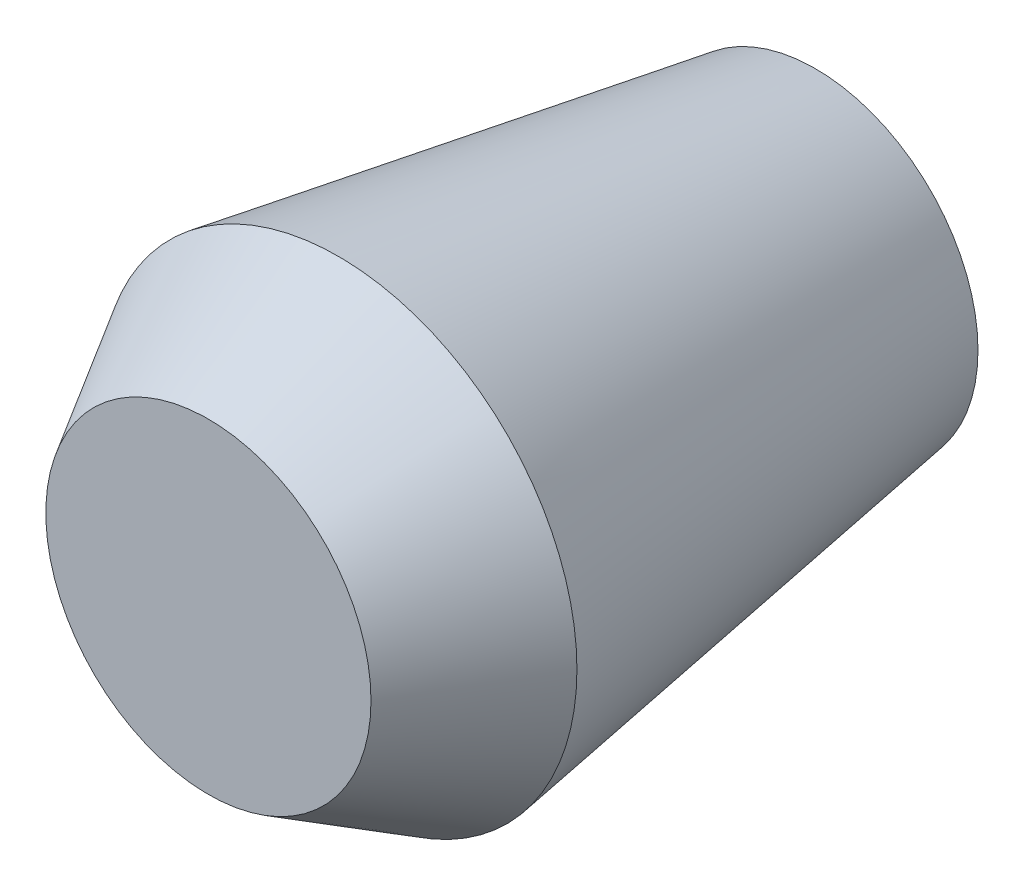
SolidWorks part; units mm, degrees
ref_plane "Front Plane" through (0, 0, 0) normal (0, 0, 1) x (1, 0, 0)
ref_plane "Top Plane" through (0, 0, 0) normal (0, 1, 0) x (1, 0, 0)
ref_plane "Right Plane" through (0, 0, 0) normal (1, 0, 0) x (0, 0, -1)
other "Configuration Table"
sketch "Sketch1" plane through (0, 0, 0) normal (0, 1, 0) x (1, 0, 0)
  line L0 (0, 0) -> (0, 44.9541) construction
  line L1 (0, 0) -> (-7.5, 0)
  line L2 (-7.5, 0) -> (-11, 6)
  line L3 (-11, 6) -> (-7.5, 28)
  line L4 (-7.5, 28) -> (0, 28)
  line L5 (0, 28) -> (0, 0)
  dimension "D1" = 28
  dimension "D2" = 7.5
  dimension "D3" = 22
  dimension "D4" = 15
  dimension "D5" = 6
revolve "Revolve1" add sketch "Sketch1" angle 360 about L0
hole_wizard "M6 Tapped Hole1" positions "Sketch2" profile "Sketch3" tap size "M6" standard "GB"
sketch "Sketch2" plane through (0, 0, -28) normal (0, 0, -1) x (-1, 0, 0)
  point P0 (0, 0)
sketch "Sketch3" plane through (0, 0, -28) normal (1, 0, 0) x (0, 1, 0)
  line L0 (0, 0) -> (0, 21.5022)
  line L1 (0, 21.5022) -> (2.5, 20)
  line L2 (2.5, 20) -> (2.5, 0)
  line L5 (2.5, 0) -> (0, 0)
  line L10 (0, 21.5022) -> (-2.5, 20) construction
  line L11 (0, -6.35) -> (0, 107.95) construction
  dimension "螺纹孔钻头直径" = 5
  dimension "螺纹孔钻头深度" = 20
  dimension "导头角度" = 118
cosmetic thread "Hole thread line2"
